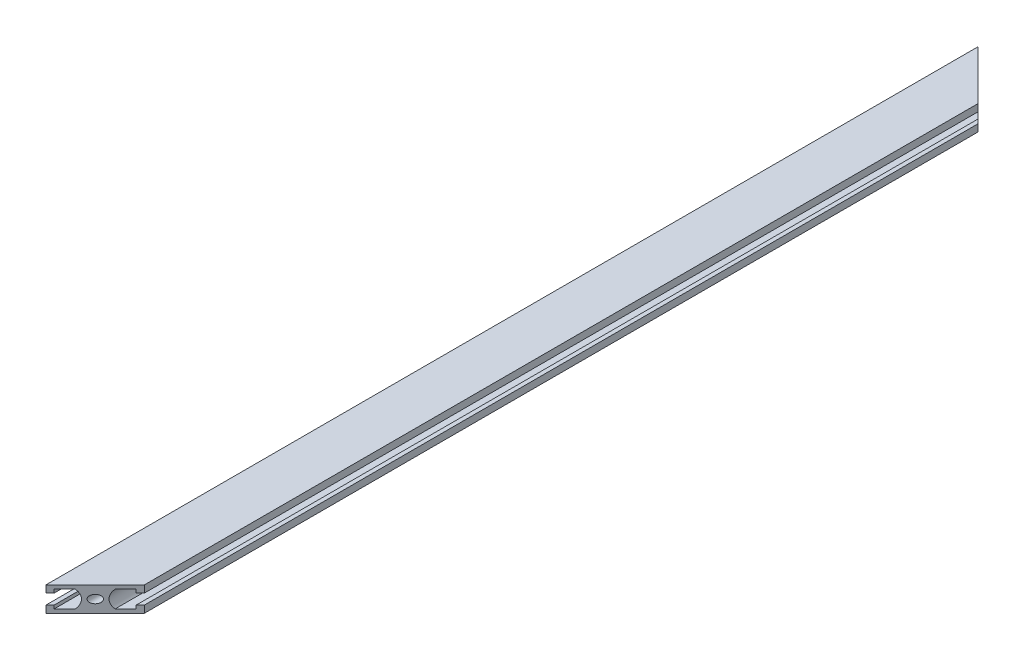
SolidWorks part; units mm, degrees
material "铝型材"
ref_plane "前视基准面" through (0, 0, 0) normal (0, 0, 1) x (1, 0, 0)
ref_plane "上视基准面" through (0, 0, 0) normal (0, 1, 0) x (1, 0, 0)
ref_plane "右视基准面" through (0, 0, 0) normal (1, 0, 0) x (0, 0, -1)
sketch "Model" plane through (0, 0, 0) normal (0, 0, 1) x (1, 0, 0)
  line L0 (2390.4271, 419.7568) -> (2392.9271, 419.7568)
  line L1 (2390.4271, 419.7568) -> (2390.4271, 417.7068)
  line L2 (2392.9271, 415.4068) -> (2392.9271, 419.7568)
  line L3 (2383.9948, 417.7068) -> (2390.4271, 417.7068)
  line L4 (2362.9271, 415.4068) -> (2392.9271, 415.4068)
  line L5 (2362.9271, 415.4068) -> (2362.9271, 419.7568)
  line L6 (2383.9948, 428.1068) -> (2390.4271, 428.1068)
  line L7 (2365.4271, 419.7568) -> (2362.9271, 419.7568)
  line L8 (2390.4271, 426.0568) -> (2390.4271, 428.1068)
  line L9 (2365.4271, 419.7568) -> (2365.4271, 417.7068)
  line L10 (2390.4271, 426.0568) -> (2392.9271, 426.0568)
  line L11 (2365.4271, 417.7068) -> (2371.8571, 417.7068)
  line L12 (2392.9271, 430.4068) -> (2392.9271, 426.0568)
  line L13 (2362.9271, 430.4068) -> (2392.9271, 430.4068)
  line L14 (2365.4271, 428.1068) -> (2371.8571, 428.1068)
  line L15 (2362.9271, 430.4068) -> (2362.9271, 426.0568)
  line L16 (2365.4271, 426.0568) -> (2365.4271, 428.1068)
  line L17 (2365.4271, 426.0568) -> (2362.9271, 426.0568)
  line L22 (2361.3714, 422.9068) -> (2394.2123, 422.9068) construction
  line L23 (2377.9271, 430.4068) -> (2377.9271, 415.4068) construction
  arc A0 (2371.8571, 428.1068) -> (2371.8571, 417.7068) centre (2365.5621, 422.9068) cw
  arc A1 (2383.9948, 428.1068) -> (2383.9948, 417.7068) centre (2390.2996, 422.9068) ccw
  circle A4 centre (2377.9271, 422.9068) radius 2.5
  point P2 (2373.7271, 422.9068)
  point P3 (2382.1271, 422.9068)
  dimension "D3" = 4.2
  dimension "D8" = 5
  dimension "D12" = 4.2
  dimension "D1" = 30
  dimension "D2" = 2.5
  dimension "D4" = 6.43
  dimension "D5" = 6.3
  dimension "D6" = 10.4
  dimension "D7" = 15
  dimension "D9" = 6.3
  dimension "D10" = 2.5
  dimension "D11" = 6.4323
extrude "凸台-拉伸1" add sketch "Model" along normal mid plane 568 contours L13 L12 L10 L8 L6 A1 L3 L1 L0 L2 L4 L5 L7 L9 L11 A0 L14 L16 L17 L15 | A4
ref_plane "基准面1" through (2382.1271, 0, 0) normal (1, 0, 0) x (0, 0, -1)
ref_plane "基准面2" through (2373.7271, 0, 0) normal (-1, 0, 0) x (0, 0, 1)
ref_plane "基准面3" through (0, 422.9068, 0) normal (0, 1, 0) x (1, 0, 0)
ref_plane "基准面4" through (2377.9271, 0, 0) normal (-1, 0, 0) x (0, 0, 1)
sketch "草图1" plane through (0, 430.4068, 0) normal (0, 1, 0) x (1, 0, 0)
  line L0 (2362.9271, 284) -> (2392.9271, 254)
  line L1 (2392.9271, -284) -> (2392.9271, 284) construction
  line L2 (2392.9271, 254) -> (2392.9271, 284)
  line L3 (2392.9271, 284) -> (2362.9271, 284)
  line L4 (2362.9271, -284) -> (2392.9271, -254)
  line L5 (2392.9271, -254) -> (2392.9271, -284)
  line L6 (2392.9271, -284) -> (2362.9271, -284)
extrude "切除-拉伸1" cut sketch "草图1" against normal through all
hole_wizard "M4 螺纹孔1" positions "草图2" profile "草图3" tap size "M4" standard "GB"
sketch "草图2" plane through (0, 415.4068, 0) normal (0, -1, 0) x (-1, 0, 0)
  line L1 (-2362.9271, -284) -> (-2362.9271, 284) construction
  line L2 (-2362.9271, 0) -> (-2453.8371, 0) construction
  point P0 (-2377.9271, -219)
  point P2 (-2377.9271, -191)
  point P4 (-2377.9271, 191)
  point P6 (-2377.9271, 219)
  dimension "D1" = 65
  dimension "D2" = 28
  dimension "D3" = 15
sketch "草图3" plane through (2377.9271, 415.4068, 219) normal (1, 0, 0) x (0, 0, -1)
  line L0 (0, 0) -> (0, 12.4914)
  line L1 (0, 12.4914) -> (1.65, 11.5)
  line L2 (1.65, 11.5) -> (1.65, 0)
  line L5 (1.65, 0) -> (0, 0)
  line L10 (0, 12.4914) -> (-1.65, 11.5) construction
  line L11 (0, -6.35) -> (0, 107.95) construction
  dimension "螺纹孔钻头直径" = 3.3
  dimension "螺纹孔钻头深度" = 11.5
  dimension "导头角度" = 118
cosmetic thread "孔螺蚊线1" parameters "D1"=8, "D2"=4
cosmetic thread "孔螺蚊线2" parameters "D1"=8, "D2"=4
cosmetic thread "孔螺蚊线3" parameters "D1"=8, "D2"=4
cosmetic thread "孔螺蚊线4" parameters "D1"=8, "D2"=4
